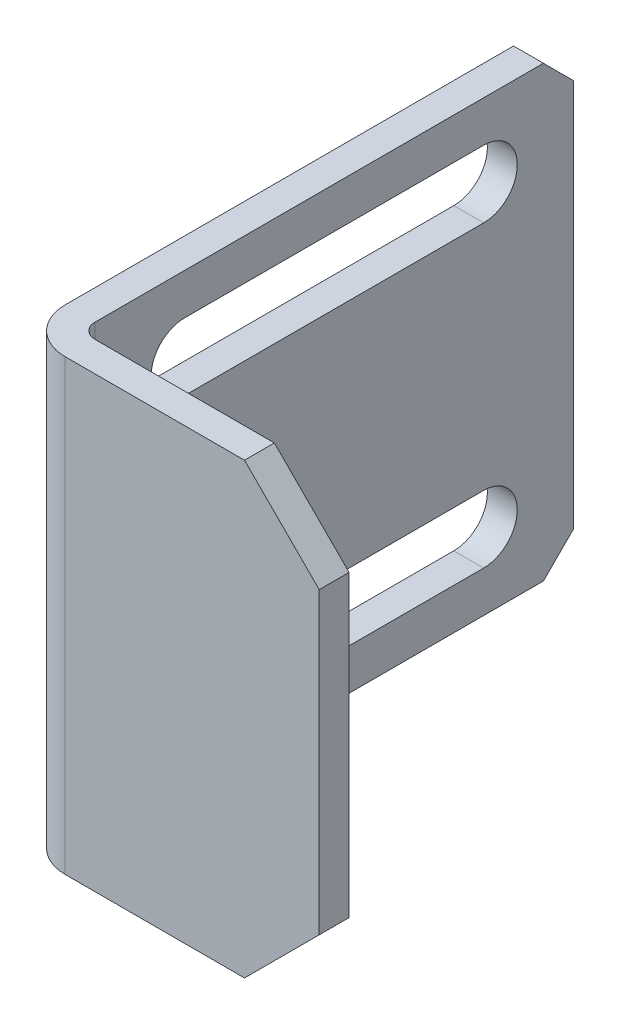
SolidWorks part; units mm, degrees
ref_plane "Front Plane" through (0, 0, 0) normal (0, 0, 1) x (1, 0, 0)
ref_plane "Top Plane" through (0, 0, 0) normal (0, 1, 0) x (1, 0, 0)
ref_plane "Right Plane" through (0, 0, 0) normal (1, 0, 0) x (0, 0, -1)
sketch "Sketch1" plane through (0, 0, 0) normal (0, 1, 0) x (1, 0, 0)
  line L1 (0, 0) -> (20, 0)
  line L2 (0, 0) -> (0, 35)
  line L3 (0, 35) -> (2, 35)
  line L4 (20, 0) -> (20, 2)
  line L7 (20, 2) -> (2, 2)
  line L8 (2, 35) -> (2, 2)
  dimension "D1" = 2
  dimension "D2" = 2
  dimension "D3" = 20
  dimension "D4" = 35
extrude "Boss-Extrude1" add sketch "Sketch1" along normal blind 30
sketch "Sketch3" plane through (2, 0, 0) normal (1, 0, 0) x (0, 0, -1)
  line L0 (0, 15) -> (50000, 15) construction
  line L1 (0, 30) -> (0, 0) construction
  line L2 (35, 30) -> (35, 0) construction
  circle A0 centre (29, 25) radius 2.25
  circle A1 centre (29, 5) radius 2.25
  point P4 (0, 15)
  dimension "D1" = 20
  dimension "D2" = 6
  dimension "D3" = 4.5
extrude "Cut-Extrude2" cut sketch "Sketch3" against normal blind 10
chamfer "Chamfer2" distance 2 angle 45 2 edges at (1, 30, -35) (1, 0, -35)
fillet "Fillet1" radius 1 1 edges at (2, 15, -2)
fillet "Fillet2" radius 3 1 edges at (0, 15, 0)
chamfer "Chamfer3" distance 5 angle 45 2 edges at (20, 30, -1) (20, 0, -1)
sketch "Sketch4" plane through (2, 0, 0) normal (1, 0, 0) x (0, 0, -1)
  line L0 (29, 5) -> (9, 5) construction
  line L1 (29, 2.75) -> (9, 2.75)
  line L2 (29, 7.25) -> (9, 7.25)
  line L3 (25, 15) -> (50025, 15) construction
  line L4 (35, 28) -> (35, 2) construction
  line L5 (29, 25) -> (9, 25) construction
  line L6 (29, 27.25) -> (9, 27.25)
  line L7 (29, 22.75) -> (9, 22.75)
  arc A0 (29, 2.75) -> (29, 7.25) centre (29, 5) ccw
  arc A1 (9, 7.25) -> (9, 2.75) centre (9, 5) ccw
  arc A2 (29, 27.25) -> (29, 22.75) centre (29, 25) cw
  arc A3 (9, 22.75) -> (9, 27.25) centre (9, 25) cw
  circle A4 centre (29, 25) radius 2.25 construction
  point P3 (19, 5)
  point P12 (35, 15)
  point P15 (19, 25)
  dimension "D1" = 20
extrude "Cut-Extrude3" cut sketch "Sketch4" against normal blind 10
